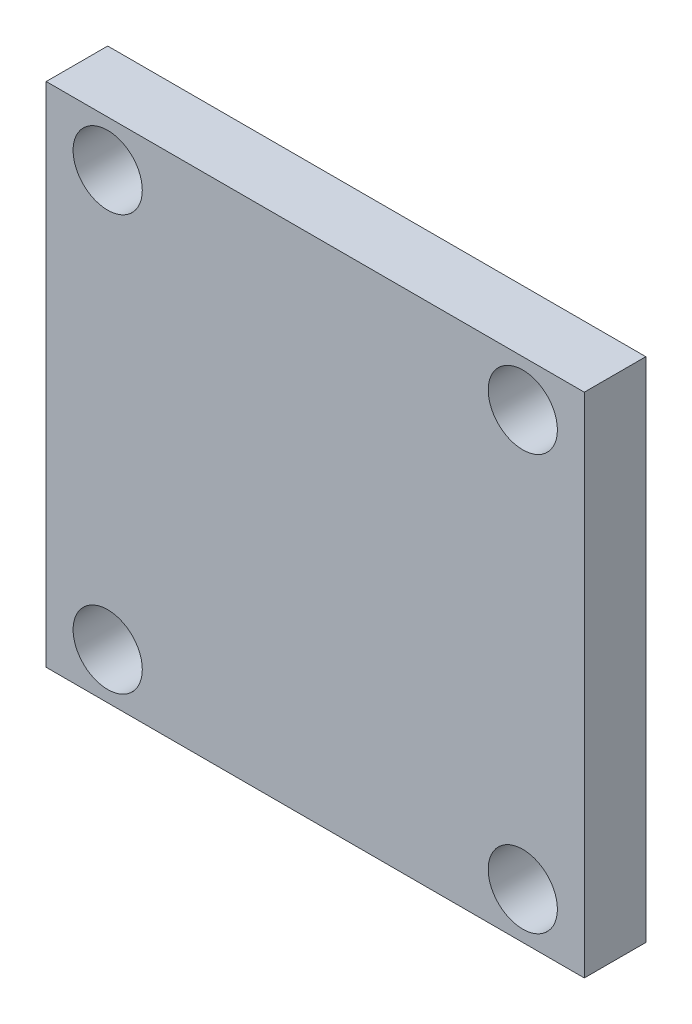
SolidWorks part; units mm, degrees
ref_plane "Front Plane" through (0, 0, 0) normal (0, 0, 1) x (1, 0, 0)
ref_plane "Top Plane" through (0, 0, 0) normal (0, 1, 0) x (1, 0, 0)
ref_plane "Right Plane" through (0, 0, 0) normal (1, 0, 0) x (0, 0, -1)
sketch "Sketch1" plane through (0, 0, 0) normal (0, 0, 1) x (1, 0, 0)
  line L1 (-17.5, 16.5) -> (17.5, 16.5)
  line L2 (-17.5, 16.5) -> (-17.5, -16.5)
  line L3 (-17.5, -16.5) -> (17.5, -16.5)
  line L4 (17.5, 16.5) -> (17.5, -16.5)
  line L5 (-17.5, 16.5) -> (17.5, -16.5) construction
  line L6 (-17.5, -16.5) -> (17.5, 16.5) construction
  point P0 (0, 0)
  dimension "D1" = 35
  dimension "D2" = 33
extrude "Boss-Extrude1" add sketch "Sketch1" along normal blind 4
hole_wizard "M4 Clearance Hole1" positions "Sketch2" profile "Sketch3" hole size "M4" standard "GB"
sketch "Sketch2" plane through (0, 0, 4) normal (0, 0, 1) x (1, 0, 0)
  line L0 (0, 0) -> (0, 21.3578) construction
  line L4 (0, 0) -> (12.2521, 0) construction
  line L6 (17.5, -16.5) -> (17.5, 16.5) construction
  line L7 (17.5, 16.5) -> (-17.5, 16.5) construction
  point P2 (13.5, 13.5)
  point P26 (-13.5, 13.5)
  point P27 (-13.5, -13.5)
  point P28 (13.5, -13.5)
  dimension "D1" = 4
  dimension "D2" = 3
sketch "Sketch3" plane through (13.5, 13.5, 4) normal (1, 0, 0) x (0, -1, 0)
  line L0 (0, 0) -> (0, 16.3519)
  line L1 (0, 16.3519) -> (2.25, 15)
  line L2 (2.25, 15) -> (2.25, 0)
  line L5 (2.25, 0) -> (0, 0)
  line L10 (0, 16.3519) -> (-2.25, 15) construction
  line L11 (0, -6.35) -> (0, 107.95) construction
  dimension "孔直径" = 4.5
  dimension "孔深度" = 15
  dimension "导头角度" = 118
